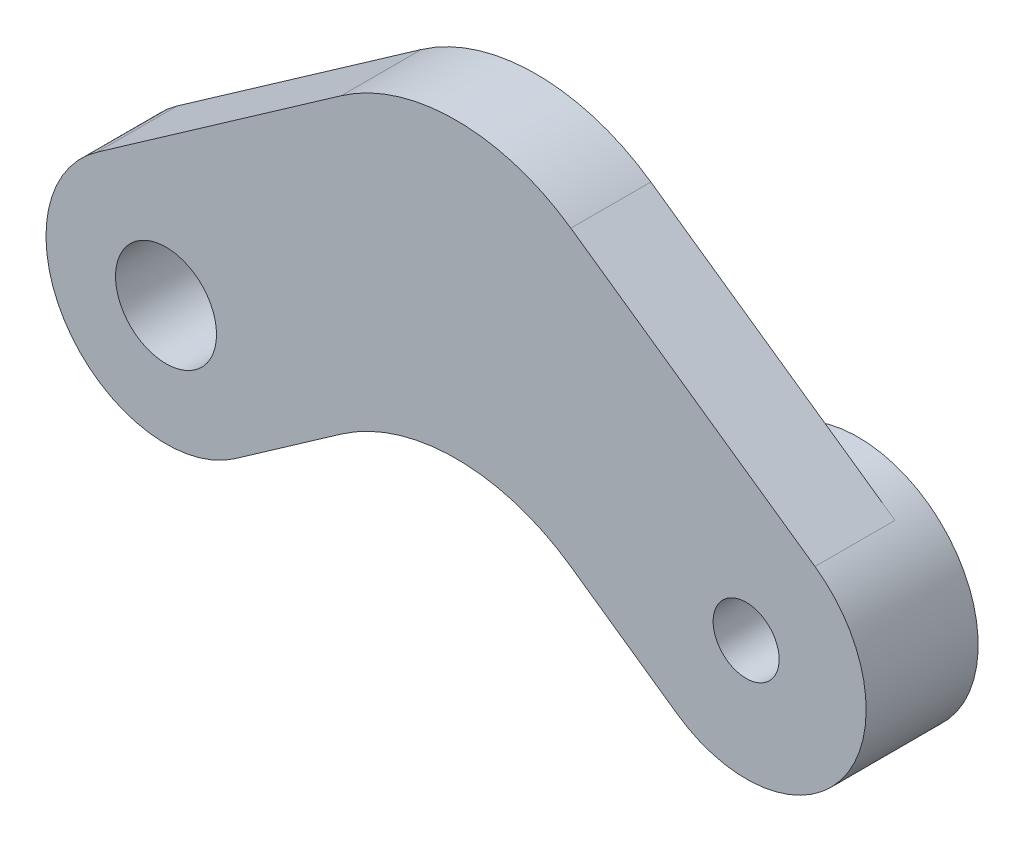
SolidWorks part; units mm, degrees
material "SKD11"
ref_plane "Front Plane" through (0, 0, 0) normal (0, 0, 1) x (1, 0, 0)
ref_plane "Top Plane" through (0, 0, 0) normal (0, 1, 0) x (1, 0, 0)
ref_plane "Right Plane" through (0, 0, 0) normal (1, 0, 0) x (0, 0, -1)
sketch "Sketch1" plane through (0, 0, 0) normal (0, 0, 1) x (1, 0, 0)
  line L0 (0, 0) -> (14.5, 10.153) construction
  line L1 (14.5, 10.153) -> (29, 0) construction
  line L2 (14.5, 2.8284) -> (14.5, -14.4617) construction
  line L3 (3.4415, -4.9149) -> (14.5, 2.8284)
  line L4 (14.5, 2.8284) -> (25.5585, -4.9149)
  line L5 (-3.4415, 4.9149) -> (14.5, 17.4777)
  line L6 (14.5, 17.4777) -> (32.4415, 4.9149)
  line L7 (17.9415, 15.0679) -> (32.4415, 4.9149) construction
  line L8 (-3.4415, 4.9149) -> (11.0585, 15.0679) construction
  line L9 (3.4415, -4.9149) -> (17.9415, 5.2381) construction
  line L10 (11.0585, 5.2381) -> (25.5585, -4.9149) construction
  arc A0 (-3.4415, 4.9149) -> (3.4415, -4.9149) centre (0, 0) ccw
  arc A1 (25.5585, -4.9149) -> (32.4415, 4.9149) centre (29, 0) ccw
  dimension "D1" = 110
  dimension "D2" = 14.5
  dimension "D3" = 6
  dimension "D6" = 6
extrude "Boss-Extrude1" add sketch "Sketch1" along normal blind 4
sketch "Sketch2" plane through (0, 0, 4) normal (0, 0, 1) x (1, 0, 0)
  circle A0 centre (0, 0) radius 2.525
  dimension "D1" = 5.05
extrude "Cut-Extrude1" cut sketch "Sketch2" against normal blind 5
sketch "Sketch7" plane through (0, 0, 0) normal (0, 0, -1) x (-1, 0, 0)
  circle A0 centre (-29, 0) radius 6
extrude "Boss-Extrude2" add sketch "Sketch7" along normal blind 1.6
hole_wizard "M4 Tapped Hole1" positions "Sketch5" profile "Sketch6" tap size "M4" standard "ISO" end condition through all
sketch "Sketch5" plane through (0, 0, 4) normal (0, 0, 1) x (1, 0, 0)
  point P0 (29, 0)
sketch "Sketch6" plane through (29, 0, 4) normal (1, 0, 0) x (0, -1, 0)
  line L0 (0, 0) -> (0, 5.6)
  line L1 (0, 5.6) -> (1.65, 5.6)
  line L2 (1.65, 5.6) -> (1.65, 0)
  line L5 (1.65, 0) -> (0, 0)
  line L11 (0, -6.35) -> (0, 107.95) construction
  dimension "通孔螺纹孔钻头直径" = 3.3
  dimension "通孔螺纹孔钻头深度" = 5.6
cosmetic thread "Cosmetic thread1"
fillet "Fillet1" radius 10 2 edges at (14.5, 17.4777, 2) (14.5, 2.8284, 2)
